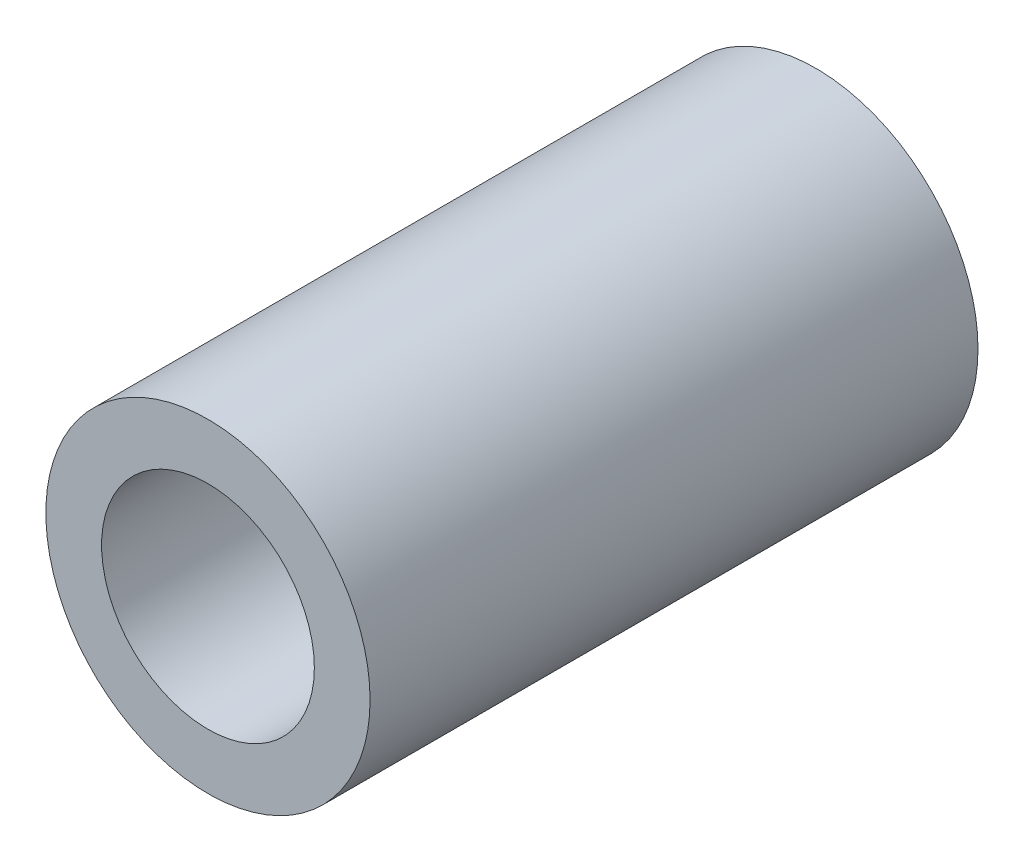
SolidWorks part; units mm, degrees
material "20"
ref_plane "Front Plane" through (0, 0, 0) normal (0, 0, 1) x (1, 0, 0)
ref_plane "Top Plane" through (0, 0, 0) normal (0, 1, 0) x (1, 0, 0)
ref_plane "Right Plane" through (0, 0, 0) normal (1, 0, 0) x (0, 0, -1)
sketch "Sketch1" plane through (0, 0, 0) normal (0, 0, 1) x (1, 0, 0)
  circle A0 centre (0, 0) radius 8
  dimension "D1" = 16
extrude "Boss-Extrude1" add sketch "Sketch1" along normal blind 30
hole_wizard "M12x1.25 Tapped Hole1" positions "Sketch3" profile "Sketch2" tap size "M12x1.25" standard "GB"
sketch "Sketch3" plane through (0, 0, 30) normal (0, 0, 1) x (1, 0, 0)
  point P0 (0, 0)
sketch "Sketch2" plane through (0, 0, 30) normal (1, 0, 0) x (0, -1, 0)
  line L0 (0, 0) -> (0, 33.1545)
  line L1 (0, 33.1545) -> (5.25, 30)
  line L2 (5.25, 30) -> (5.25, 0)
  line L5 (5.25, 0) -> (0, 0)
  line L10 (0, 33.1545) -> (-5.25, 30) construction
  line L11 (0, -6.35) -> (0, 107.95) construction
  dimension "螺纹孔钻头直径" = 10.5
  dimension "螺纹孔钻头深度" = 30
  dimension "导头角度" = 118
cosmetic thread "Cosmetic thread2" parameters "D1"=20, "D2"=12
